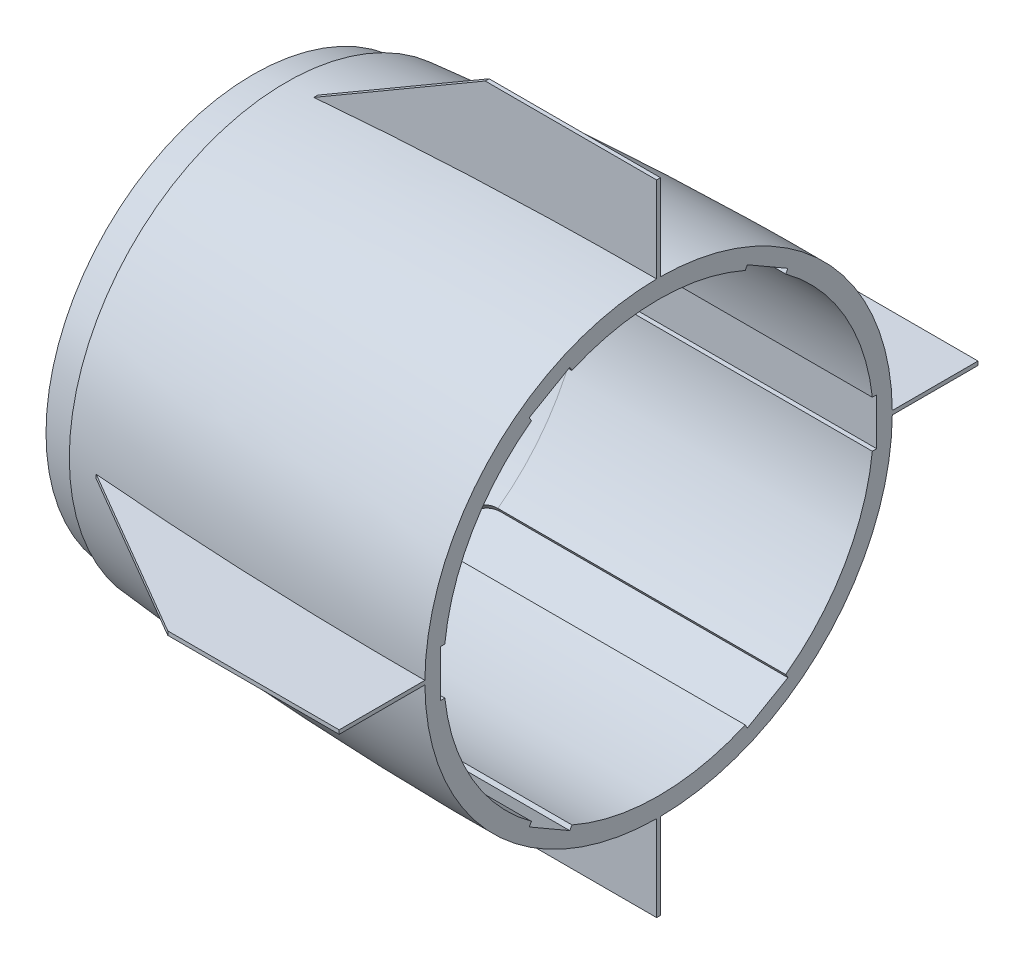
SolidWorks part; units mm, degrees
other "Camera1"
material "ABS"
ref_plane "Front Plane" through (0, 0, 0) normal (0, 0, 1) x (1, 0, 0)
ref_plane "Top Plane" through (0, 0, 0) normal (0, 1, 0) x (1, 0, 0)
ref_plane "Right Plane" through (0, 0, 0) normal (1, 0, 0) x (0, 0, -1)
sketch "Sketch1" plane through (0, 0, 0) normal (0, 0, 1) x (1, 0, 0)
  line L0 (735.5722, 1570.5269) -> (3256.9057, 1570.5269) construction
  line L1 (86, 109.4852) -> (430, 109.4852) construction
  line L2 (0, 0) -> (665, 0) construction
  line L3 (0, 0) -> (0, 300) construction
  line L4 (0, 300) -> (665, 300) construction
  line L5 (665, 0) -> (665, 300) construction
  line L6 (665, 300) -> (733.25, 300) construction
  line L7 (733.25, 300) -> (733.25, 0) construction
  line L8 (733.25, 0) -> (665, 0) construction
  dimension "D1" = 665
  dimension "D2" = 300
  dimension "D3" = 68.25
  dimension "D4" = 733.25
sketch "Sketch2" plane through (0, 0, 0) normal (0, 0, 1) x (1, 0, 0)
  line L0 (0, 150) -> (748.2165, 150) construction
  line L1 (0, 0) -> (0, 300) construction
  line L2 (227.8403, 235.5893) -> (227.8403, 205.0425)
  line L3 (0, 150) -> (11.0244, 150)
  line L4 (11.0244, 150) -> (11.0244, 162.723)
  line L5 (11.0244, 162.723) -> (16.7389, 162.723)
  line L6 (16.7389, 162.723) -> (16.7389, 168.0858)
  line L7 (16.7389, 168.0858) -> (23.7721, 168.0858)
  line L8 (23.7721, 168.0858) -> (23.7721, 170.987)
  line L9 (23.7721, 170.987) -> (31.3328, 170.987)
  line L10 (31.3328, 170.987) -> (31.3328, 175.2948)
  line L11 (31.3328, 175.2948) -> (36.9593, 175.2948)
  line L12 (36.9593, 175.2948) -> (36.9593, 177.6685)
  line L13 (36.9593, 177.6685) -> (43.8167, 177.6685)
  line L14 (43.8167, 177.6685) -> (43.8167, 180.7455)
  line L15 (43.8167, 180.7455) -> (50.9378, 180.7455)
  line L16 (50.9378, 180.7455) -> (50.9378, 184.6138)
  line L17 (50.9378, 184.6138) -> (63.5975, 184.6138)
  line L18 (63.5975, 184.6138) -> (63.5975, 189.1854)
  line L19 (63.5975, 189.1854) -> (76.6089, 189.1854)
  line L20 (76.6089, 189.1854) -> (76.6089, 192.2624)
  line L21 (76.6089, 192.2624) -> (90.1478, 192.2624)
  line L22 (90.1478, 192.2624) -> (90.1478, 195.1804)
  line L23 (90.1478, 195.1804) -> (102.9206, 195.1804)
  line L24 (102.9206, 195.1804) -> (102.9206, 205.0425)
  line L25 (11.0244, 150) -> (0, 150)
  line L26 (214.5353, 237.8889) -> (227.8403, 235.5893)
  line L27 (227.8403, 235.5893) -> (227.8403, 241.0099)
  line L28 (227.8403, 241.0099) -> (247.1953, 246.2894)
  line L29 (247.1953, 246.2894) -> (247.1953, 251.0437)
  line L30 (227.8403, 205.0425) -> (241.4162, 209.4748)
  line L31 (241.4162, 209.4748) -> (241.4162, 232.1247)
  line L32 (241.4162, 232.1247) -> (249.4192, 232.1247)
  line L33 (249.4192, 232.1247) -> (249.4192, 241.0099)
  line L34 (249.4192, 241.0099) -> (259.5362, 248.5837)
  line L35 (420.7962, 276.5625) -> (429.255, 273.4621)
  line L36 (429.255, 273.4621) -> (429.255, 277.7797)
  line L37 (548.5551, 288.0038) -> (733.25, 288.0038)
  line L38 (733.25, 300) -> (733.25, 0) construction
  line L39 (733.25, 288.0038) -> (733.25, 300)
  line L40 (450.638, 280.4227) -> (450.638, 284.7325)
  line L41 (429.255, 273.4621) -> (452.5798, 276.5625)
  line L42 (452.5798, 276.5625) -> (456.4938, 281.0865)
  arc A0 (14.2697, 172.5801) -> (0, 150) centre (25, 150) ccw
  spline S0 degree 3 poles (14.2697, 172.5801) (42.76, 186.119) (109.5451, 213.865) (336.1702, 281.43) (571.9418, 300.1185) (733.25, 300) knots 0 0 0 0 0.115606 0.303282 1 1 1 1
  spline S1 degree 2 poles (102.9206, 205.0425) (158.2549, 224.3358) (214.5353, 237.8889) knots 0 0 0 1 1 1
  spline S2 degree 2 poles (259.5362, 248.5837) (339.3196, 266.0447) (420.7962, 276.5625) knots 0 0 0 1 1 1
  spline S3 degree 3 poles (429.255, 277.7797) (436.4066, 278.7206) (443.5343, 279.6016) (450.638, 280.4227) knots 0 0 0 0 0.176421 0.176421 0.176421 0.176421
  spline S4 degree 2 poles (456.4938, 281.0865) (503.2189, 286.28) (548.5551, 288.0038) knots 0.224943 0.224943 0.224943 1 1 1
  dimension "D1" = 50
revolve "Revolve3" add sketch "Sketch2" angle 360 about L0
ref_plane "Plane2" through (460, 0, 0) normal (1, 0, 0) x (0, 0, -1)
ref_plane "Plane3" through (0, 150, 0) normal (0, 1, 0) x (1, 0, 0)
sketch "Sketch5" plane through (0, 0, 0) normal (0, 0, 1) x (1, 0, 0)
  line L0 (548.5551, 288.0038) -> (548.5551, 11.9962) construction
  line L1 (548.5551, 165) -> (733.25, 165)
  line L2 (733.25, 11.9962) -> (733.25, 288.0038) construction
  line L3 (733.25, 165) -> (733.25, 135)
  line L4 (733.25, 135) -> (548.5551, 135)
  arc A0 (548.5551, 165) -> (548.5551, 135) centre (548.5551, 150) ccw
  dimension "D1" = 30
extrude "Cut-Extrude1" cut sketch "Sketch5" against normal blind 140
pattern_circular "CirPattern3" count 6 over 360 about axis through (0, 150, 0) along (1, 0, 0) of "Cut-Extrude1"
sketch "Sketch6" plane through (0, 0, 0) normal (0, 0, 1) x (1, 0, 0)
  line L0 (733.25, 297.5) -> (733.25, 355)
  line L1 (733.25, 355) -> (623.25, 355)
  line L2 (623.25, 355) -> (513.25, 290.9011)
  line L3 (513.25, 290.9011) -> (733.25, 297.5)
  line L4 (733.25, 0) -> (733.25, 300) construction
  spline S0 degree 3 poles (733.25, 300) (643.914, 300.0656) (547.0845, 295.5792) (450.638, 284.7325) knots 0 0 0 0 0.385858 0.385858 0.385858 0.385858 construction
  dimension "D1" = 28.512
  dimension "D2" = 55
  dimension "D3" = 110
  dimension "D4" = 220
  dimension "D5" = 2.5
extrude "Boss-Extrude2" add sketch "Sketch6" along normal mid plane 2.5
pattern_circular "CirPattern5" count 4 over 360 about axis through (0, 150, 0) along (1, 0, 0) of "Boss-Extrude2"
ref_axis "Axis1" through (733.25, 150, 0) along (-1, 0, 0)
sketch "Sketch7" plane through (0, 0, 0) normal (0, 0, 1) x (1, 0, 0)
  line L0 (494.255, 301.9537) -> (494.255, -12.4523)
  line L1 (429.255, 277.7797) -> (429.255, 22.2203) construction
  line L2 (429.4724, -12.4523) -> (429.4724, 301.9537)
  line L3 (429.4724, 301.9537) -> (494.255, 301.9537)
  line L4 (494.255, -12.4523) -> (429.4724, -12.4523)
  dimension "D1" = 65
extrude "Cut-Extrude2" cut sketch "Sketch7" against normal blind 160 and the other way blind 140
sketch "Sketch8" plane through (0, 0, 0) normal (0, 0, 1) x (1, 0, 0)
  line L1 (494.255, 289.2105) -> (494.255, 10.7895) construction
  line L2 (494.255, 284.7358) -> (494.255, 15.2642) construction
  line L3 (500.0137, 285.1598) -> (500.0137, 287.9375)
  line L4 (494.255, 287.4922) -> (500.0137, 287.9375)
  line L35 (472.9517, 278.091) -> (472.9517, 282.8527)
  line L38 (494.255, 284.7358) -> (494.255, 287.4922)
  line L39 (472.9517, 278.091) -> (495.8114, 280.4785)
  line L40 (495.8114, 280.4785) -> (500.0137, 285.1598)
  spline S3 degree 3 poles (472.9517, 282.8527) (480.1033, 283.7937) (487.1513, 283.9147) (494.255, 284.7358) knots 0 0 0 0 0.176421 0.176421 0.176421 0.176421
revolve "Revolve4" add sketch "Sketch8" angle 360 about axis through (733.25, 150, 0) along (-1, 0, 0)
